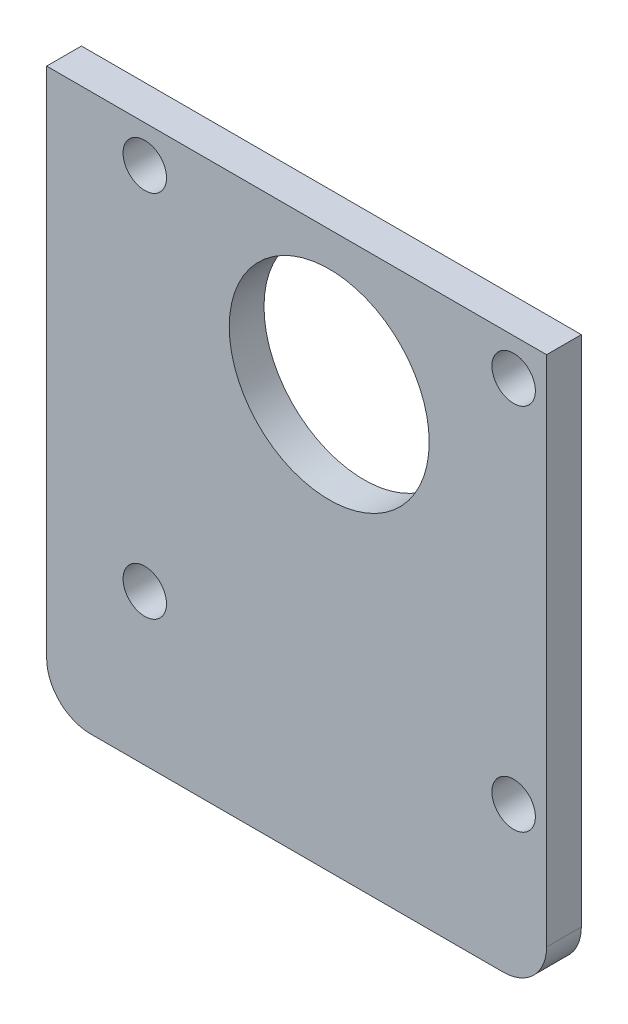
SolidWorks part; units mm, degrees
material "Q235B"
ref_plane "Front Plane" through (0, 0, 0) normal (0, 0, 1) x (1, 0, 0)
ref_plane "Top Plane" through (0, 0, 0) normal (0, 1, 0) x (1, 0, 0)
ref_plane "Right Plane" through (0, 0, 0) normal (1, 0, 0) x (0, 0, -1)
sketch "Sketch1" plane through (0, 0, 0) normal (0, 0, 1) x (1, 0, 0)
  line L1 (57.5, -64) -> (-57.5, -64)
  line L2 (57.5, -64) -> (57.5, 64)
  line L3 (57.5, 64) -> (-57.5, 64)
  line L4 (-57.5, -64) -> (-57.5, 64)
  line L5 (57.5, -64) -> (-57.5, 64) construction
  line L6 (57.5, 64) -> (-57.5, -64) construction
  circle A0 centre (6.57, 34) radius 23 construction
  point P0 (0, 0)
  dimension "D3" = 46
  dimension "D4" = 50.93
  dimension "D5" = 30
  dimension "D1" = 128
  dimension "D2" = 115
extrude "Boss-Extrude1" add sketch "Sketch1" along normal mid plane 8
hole_wizard "Ø10 Hole1" positions "Sketch2" profile "Sketch3" hole size "Ø10.0" standard "GB" end condition up to next
sketch "Sketch2" plane through (0, 0, 4) normal (0, 0, 1) x (1, 0, 0)
  line L0 (7.5, 64) -> (7.5, 13.0736) construction
  line L1 (57.5, 64) -> (-57.5, 64) construction
  line L2 (7.5, 13.0736) -> (-38.1407, 13.0736) construction
  line L4 (7.5, 13.0736) -> (-34.9264, 55.5) construction
  line L5 (57.5, -64) -> (57.5, 64) construction
  circle A1 centre (7.5, 13.0736) radius 60
  point P0 (-34.9264, 55.5)
  point P13 (49.9264, 55.5)
  point P14 (49.9264, -29.3528)
  point P15 (-34.9264, -29.3528)
  dimension "D1" = 120
  dimension "D2" = 45
  dimension "D3" = 8.5
  dimension "D4" = 50
sketch "Sketch3" plane through (-34.9264, 55.5, 4) normal (1, 0, 0) x (0, -1, 0)
  line L0 (0, 0) -> (0, 8)
  line L1 (0, 8) -> (5, 8)
  line L2 (5, 8) -> (5, 0)
  line L5 (5, 0) -> (0, 0)
  line L11 (0, -6.35) -> (0, 107.95) construction
  dimension "通孔孔直径" = 10
  dimension "通孔孔深度" = 8
chamfer "Chamfer1" [suppressed] distance 10 angle 45
fillet "Fillet1" radius 10 2 edges at (57.5, -64, 0) (-57.5, -64, 0)
sketch "Sketch4" plane through (0, 0, 4) normal (0, 0, 1) x (1, 0, 0)
  line L0 (-34.9264, 55.5) -> (49.9264, 55.5) construction
  line L1 (7.5, 55.5) -> (7.5, 33.0736) construction
  circle A0 centre (7.5, 33.0736) radius 23
  dimension "D1" = 46
  dimension "D2" = 20
extrude "Cut-Extrude1" cut sketch "Sketch4" against normal up to next
